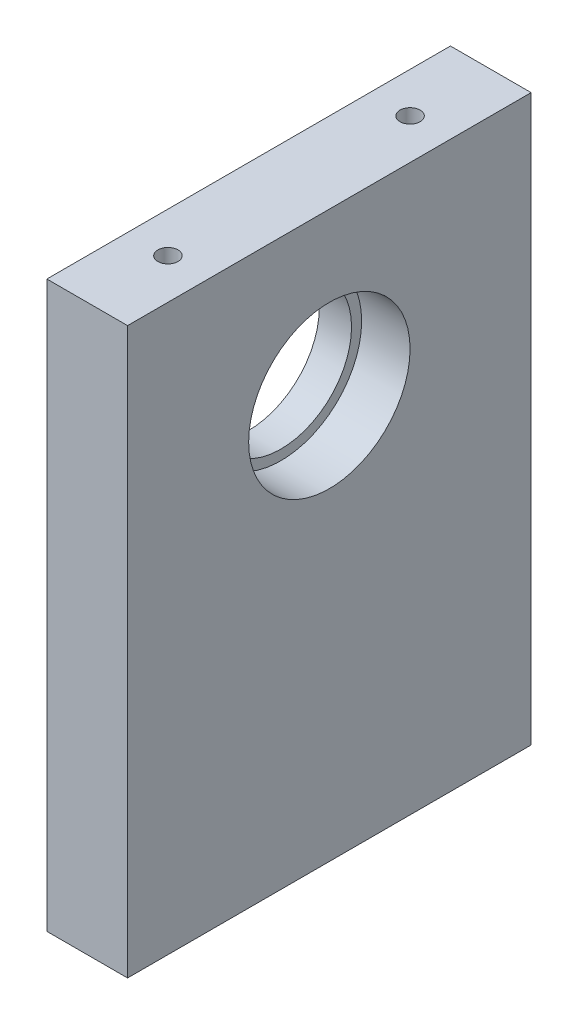
from build123d import *

# Parameters (mm, degrees)
SKETCH_1_W              = 100
SKETCH_1_H              = 140
EXTRUDE_1_DEPTH         = 20
HOLE_WIZARD_M10_1_D     = 8.5
HOLE_WIZARD_M10_1_DEPTH = 24.5
HOLE_WIZARD_M10_1_TIP   = 2.553657631
SKETCH_4_R              = 20
CUT_EXTRUDE_1_DEPTH     = 12
SKETCH_5_R              = 17.5
CUT_EXTRUDE_2_DEPTH     = 87.856203002
HOLE_WIZARD_M6_1_D      = 5
HOLE_WIZARD_M6_1_DEPTH  = 15
HOLE_WIZARD_M6_1_TIP    = 1.502151548


with BuildPart() as part:
    # 草图1 → 凸台-拉伸1 (new body)
    with BuildSketch(Plane(origin=(0, 0, 0), x_dir=(0, 0, -1), z_dir=(1, 0, 0))):
        Rectangle(SKETCH_1_W, SKETCH_1_H)
    extrude(amount=EXTRUDE_1_DEPTH)

    # M10 螺纹孔1
    with Locations(Plane(origin=(0, -70, 0), x_dir=(-1, 0, 0), z_dir=(0, -1, 0))):
        with Locations((-10, 30), (-10, -30)):
            Hole(HOLE_WIZARD_M10_1_D / 2, depth=HOLE_WIZARD_M10_1_DEPTH)
            with Locations((0, 0, -(HOLE_WIZARD_M10_1_DEPTH + HOLE_WIZARD_M10_1_TIP / 2))):  # 118° drill point
                Cone(0, HOLE_WIZARD_M10_1_D / 2, HOLE_WIZARD_M10_1_TIP, mode=Mode.SUBTRACT)

    # 草图4 → 切除-拉伸1 (cut)
    with BuildSketch(Plane(origin=(20, 0, 0), x_dir=(0, 0, -1), z_dir=(1, 0, 0))):
        with Locations((0, 30)):
            Circle(SKETCH_4_R)
    extrude(amount=-CUT_EXTRUDE_1_DEPTH, mode=Mode.SUBTRACT)

    # 草图5 → 切除-拉伸2 (cut, through all)
    with BuildSketch(Plane(origin=(8, 0, 0), x_dir=(0, 0, -1), z_dir=(1, 0, 0))):
        with Locations((0, 30)):
            Circle(SKETCH_5_R)
    extrude(amount=-CUT_EXTRUDE_2_DEPTH, mode=Mode.SUBTRACT)

    # M6 螺纹孔1
    with Locations(Plane(origin=(0, 70, 0), x_dir=(1, 0, 0), z_dir=(0, 1, 0))):
        with Locations((10, 30), (10, -30)):
            Hole(HOLE_WIZARD_M6_1_D / 2, depth=HOLE_WIZARD_M6_1_DEPTH)
            with Locations((0, 0, -(HOLE_WIZARD_M6_1_DEPTH + HOLE_WIZARD_M6_1_TIP / 2))):  # 118° drill point
                Cone(0, HOLE_WIZARD_M6_1_D / 2, HOLE_WIZARD_M6_1_TIP, mode=Mode.SUBTRACT)


solid = part.part
